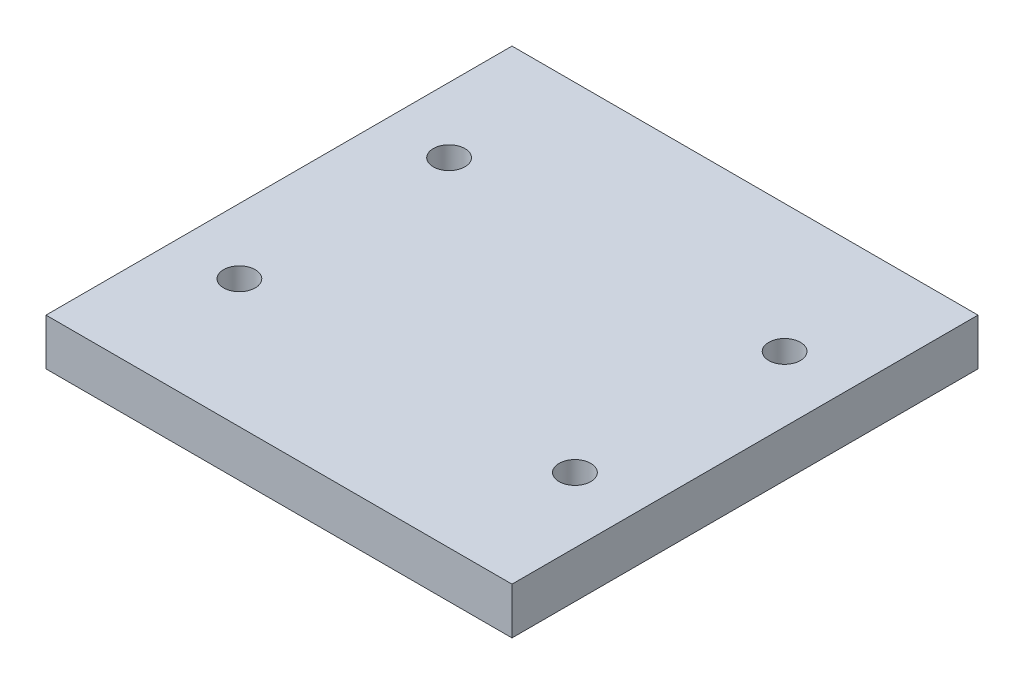
from build123d import *

# Parameters (mm, degrees)
SKETCH_1_W         = 100
SKETCH_1_H         = 100
EXTRUDE_1_DEPTH    = 10
HOLE_WIZARD_M8_1_D = 6.8


with BuildPart() as part:
    # 草图1 → 拉伸1 (new body)
    with BuildSketch(Plane(origin=(0, 0, 0), x_dir=(1, 0, 0), z_dir=(0, 1, 0))):
        Rectangle(SKETCH_1_W, SKETCH_1_H)
    extrude(amount=EXTRUDE_1_DEPTH)

    # M8 螺纹孔1 (through all)
    with Locations(Plane(origin=(-36, 0, 22.5), x_dir=(0, 0, -1), z_dir=(0, -1, 0))):
        with Locations((0, 0), (45, 0), (0, 72), (45, 72)):
            Hole(HOLE_WIZARD_M8_1_D / 2)


solid = part.part
